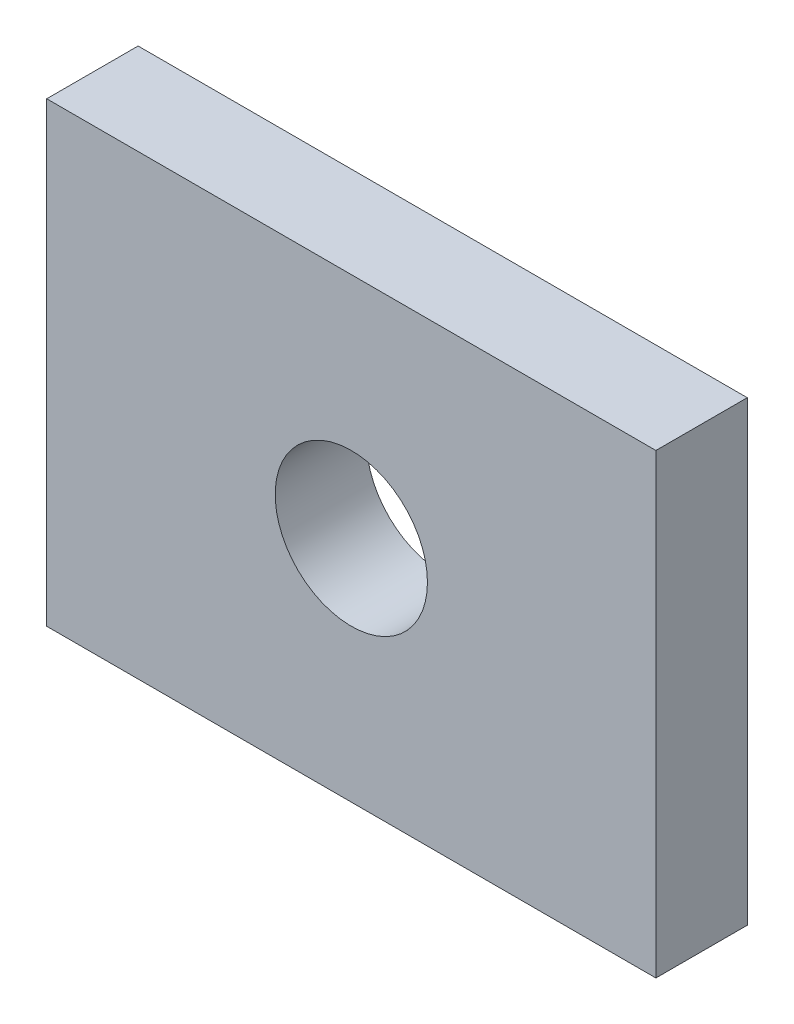
SolidWorks part; units mm, degrees
material "PBT general purpose"
ref_plane "Front Plane" through (0, 0, 0) normal (0, 0, 1) x (1, 0, 0)
ref_plane "Top Plane" through (0, 0, 0) normal (0, 1, 0) x (1, 0, 0)
ref_plane "Right Plane" through (0, 0, 0) normal (1, 0, 0) x (0, 0, -1)
sketch "Sketch1" plane through (0, 0, 0) normal (0, 0, 1) x (1, 0, 0)
  line L1 (-46.669, 11.8678) -> (-6.669, 11.8678)
  line L2 (-46.669, 11.8678) -> (-46.669, -18.1322)
  line L3 (-46.669, -18.1322) -> (-6.669, -18.1322)
  line L4 (-6.669, 11.8678) -> (-6.669, -18.1322)
extrude "Boss-Extrude1" add sketch "Sketch1" along normal blind 6
sketch "Sketch2" plane through (0, 0, 6) normal (0, 0, 1) x (1, 0, 0)
  circle A0 centre (-26.669, -3.1322) radius 5
extrude "Cut-Extrude1" cut sketch "Sketch2" against normal blind 6
